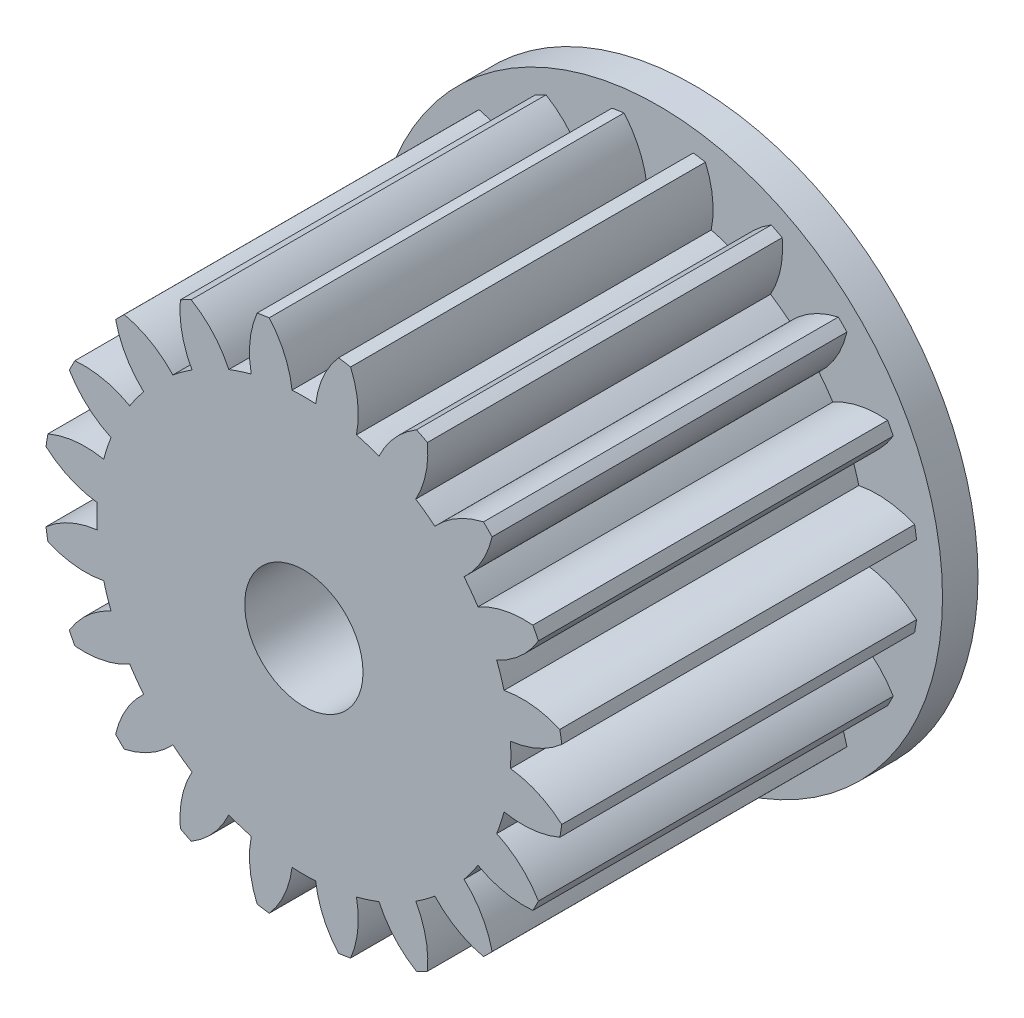
SolidWorks part; units mm, degrees
ref_plane "Front Plane" through (0, 0, 0) normal (0, 0, 1) x (1, 0, 0)
ref_plane "Top Plane" through (0, 0, 0) normal (0, 1, 0) x (1, 0, 0)
ref_plane "Right Plane" through (0, 0, 0) normal (1, 0, 0) x (0, 0, -1)
other "Configuration Table"
sketch "Sketch1" plane through (0, 0, 0) normal (0, 0, 1) x (1, 0, 0)
  circle A0 centre (0, 0) radius 12
  dimension "D1" = 24
extrude "Boss-Extrude1" add sketch "Sketch1" along normal blind 1.5
sketch "Sketch2" plane through (0, 0, 1.5) normal (0, 0, 1) x (1, 0, 0)
  arc A1 (-10.902, 1.5642) -> (-8.7347, 0.5992) centre (-8.2645, 4.5714) ccw
  arc A2 (-8.7347, 0.5992) -> (-8.7347, -0.4007) centre (0, 0.0992) ccw
  arc A3 (-8.7347, -0.4007) -> (-10.902, -1.3657) centre (-8.2645, -4.3729) ccw
  arc A4 (-10.902, -1.3657) -> (-10.8211, -1.8764) centre (0, 0.0992) ccw
  arc A5 (-10.8211, -1.8764) -> (-8.4617, -2.1245) centre (-9.242, 1.7987) ccw
  arc A6 (-8.4617, -2.1245) -> (-8.1527, -3.0754) centre (0, 0.0992) ccw
  arc A7 (-8.1527, -3.0754) -> (-9.9157, -4.6629) centre (-6.478, -6.7079) ccw
  arc A8 (-9.9157, -4.6629) -> (-9.681, -5.1236) centre (0, 0.0992) ccw
  arc A9 (-9.681, -5.1236) -> (-7.3604, -4.6304) centre (-9.3148, -1.1404) ccw
  arc A10 (-7.3604, -4.6304) -> (-6.7727, -5.4393) centre (0, 0.0992) ccw
  arc A11 (-6.7727, -5.4393) -> (-7.9588, -7.494) centre (-4.0574, -8.3766) ccw
  arc A12 (-7.9588, -7.494) -> (-7.5932, -7.8596) centre (0, 0.0992) ccw
  arc A13 (-7.5932, -7.8596) -> (-5.5386, -6.6734) centre (-8.4758, -3.9582) ccw
  arc A14 (-5.5386, -6.6734) -> (-4.7297, -7.2611) centre (0, 0.0992) ccw
  arc A15 (-4.7297, -7.2611) -> (-5.2229, -9.5817) centre (-1.2397, -9.2155) ccw
  arc A16 (-5.2229, -9.5817) -> (-4.7622, -9.8165) centre (0, 0.0992) ccw
  arc A17 (-4.7622, -9.8165) -> (-3.1746, -8.0535) centre (-6.8072, -6.3788) ccw
  arc A18 (-3.1746, -8.0535) -> (-2.2237, -8.3624) centre (0, 0.0992) ccw
  arc A19 (-2.2237, -8.3624) -> (-1.9757, -10.7219) centre (1.6994, -9.1427) ccw
  arc A20 (-1.9757, -10.7219) -> (-1.465, -10.8028) centre (0, 0.0992) ccw
  arc A21 (-1.465, -10.8028) -> (-0.4999, -8.6355) centre (-4.4722, -8.1652) ccw
  arc A22 (-0.4999, -8.6355) -> (0.4999, -8.6355) centre (0, 0.0992) ccw
  arc A23 (0.4999, -8.6355) -> (1.465, -10.8028) centre (4.4722, -8.1652) ccw
  arc A24 (1.465, -10.8028) -> (1.9757, -10.7219) centre (0, 0.0992) ccw
  arc A25 (1.9757, -10.7219) -> (2.2237, -8.3624) centre (-1.6994, -9.1427) ccw
  arc A26 (2.2237, -8.3624) -> (3.1746, -8.0535) centre (0, 0.0992) ccw
  arc A27 (3.1746, -8.0535) -> (4.7622, -9.8165) centre (6.8072, -6.3788) ccw
  arc A28 (4.7622, -9.8165) -> (5.2229, -9.5817) centre (0, 0.0992) ccw
  arc A29 (5.2229, -9.5817) -> (4.7297, -7.2611) centre (1.2397, -9.2155) ccw
  arc A30 (4.7297, -7.2611) -> (5.5386, -6.6734) centre (0, 0.0992) ccw
  arc A31 (5.5386, -6.6734) -> (7.5932, -7.8596) centre (8.4758, -3.9582) ccw
  arc A32 (7.5932, -7.8596) -> (7.9588, -7.494) centre (0, 0.0992) ccw
  arc A33 (7.9588, -7.494) -> (6.7727, -5.4393) centre (4.0574, -8.3766) ccw
  arc A34 (6.7727, -5.4393) -> (7.3604, -4.6304) centre (0, 0.0992) ccw
  arc A35 (7.3604, -4.6304) -> (9.681, -5.1236) centre (9.3148, -1.1404) ccw
  arc A36 (9.681, -5.1236) -> (9.9157, -4.6629) centre (0, 0.0992) ccw
  arc A37 (9.9157, -4.6629) -> (8.1527, -3.0754) centre (6.478, -6.7079) ccw
  arc A38 (8.1527, -3.0754) -> (8.4617, -2.1245) centre (0, 0.0992) ccw
  arc A39 (8.4617, -2.1245) -> (10.8211, -1.8764) centre (9.242, 1.7987) ccw
  arc A40 (10.8211, -1.8764) -> (10.902, -1.3657) centre (0, 0.0992) ccw
  arc A41 (10.902, -1.3657) -> (8.7347, -0.4007) centre (8.2645, -4.3729) ccw
  arc A42 (8.7347, -0.4007) -> (8.7347, 0.5992) centre (0, 0.0992) ccw
  arc A43 (8.7347, 0.5992) -> (10.902, 1.5642) centre (8.2645, 4.5714) ccw
  arc A44 (10.902, 1.5642) -> (10.8211, 2.0749) centre (0, 0.0992) ccw
  arc A45 (10.8211, 2.0749) -> (8.4617, 2.323) centre (9.242, -1.6002) ccw
  arc A46 (8.4617, 2.323) -> (8.1527, 3.2739) centre (0, 0.0992) ccw
  arc A47 (8.1527, 3.2739) -> (9.9157, 4.8614) centre (6.478, 6.9064) ccw
  arc A48 (9.9157, 4.8614) -> (9.681, 5.3221) centre (0, 0.0992) ccw
  arc A49 (9.681, 5.3221) -> (7.3604, 4.8289) centre (9.3148, 1.3389) ccw
  arc A50 (7.3604, 4.8289) -> (6.7727, 5.6378) centre (0, 0.0992) ccw
  arc A51 (6.7727, 5.6378) -> (7.9588, 7.6925) centre (4.0574, 8.5751) ccw
  arc A52 (7.9588, 7.6925) -> (7.5932, 8.0581) centre (0, 0.0992) ccw
  arc A53 (7.5932, 8.0581) -> (5.5386, 6.8719) centre (8.4758, 4.1567) ccw
  arc A54 (5.5386, 6.8719) -> (4.7297, 7.4596) centre (0, 0.0992) ccw
  arc A55 (4.7297, 7.4596) -> (5.2229, 9.7802) centre (1.2397, 9.414) ccw
  arc A56 (5.2229, 9.7802) -> (4.7622, 10.015) centre (0, 0.0992) ccw
  arc A57 (4.7622, 10.015) -> (3.1746, 8.252) centre (6.8072, 6.5773) ccw
  arc A58 (3.1746, 8.252) -> (2.2237, 8.5609) centre (0, 0.0992) ccw
  arc A59 (2.2237, 8.5609) -> (1.9757, 10.9204) centre (-1.6994, 9.3412) ccw
  arc A60 (1.9757, 10.9204) -> (1.465, 11.0013) centre (0, 0.0992) ccw
  arc A61 (1.465, 11.0013) -> (0.4999, 8.834) centre (4.4722, 8.3637) ccw
  arc A62 (0.4999, 8.834) -> (-0.4999, 8.834) centre (0, 0.0992) ccw
  arc A63 (-0.4999, 8.834) -> (-1.465, 11.0013) centre (-4.4722, 8.3637) ccw
  arc A64 (-1.465, 11.0013) -> (-1.9757, 10.9204) centre (0, 0.0992) ccw
  arc A65 (-1.9757, 10.9204) -> (-2.2237, 8.5609) centre (1.6994, 9.3412) ccw
  arc A66 (-2.2237, 8.5609) -> (-3.1746, 8.252) centre (0, 0.0992) ccw
  arc A67 (-3.1746, 8.252) -> (-4.7622, 10.015) centre (-6.8072, 6.5773) ccw
  arc A68 (-4.7622, 10.015) -> (-5.2229, 9.7802) centre (0, 0.0992) ccw
  arc A69 (-5.2229, 9.7802) -> (-4.7297, 7.4596) centre (-1.2397, 9.414) ccw
  arc A70 (-4.7297, 7.4596) -> (-5.5386, 6.8719) centre (0, 0.0992) ccw
  arc A71 (-5.5386, 6.8719) -> (-7.5932, 8.0581) centre (-8.4758, 4.1567) ccw
  arc A72 (-7.5932, 8.0581) -> (-7.9588, 7.6925) centre (0, 0.0992) ccw
  arc A73 (-7.9588, 7.6925) -> (-6.7727, 5.6378) centre (-4.0574, 8.5751) ccw
  arc A74 (-6.7727, 5.6378) -> (-7.3604, 4.8289) centre (0, 0.0992) ccw
  arc A75 (-7.3604, 4.8289) -> (-9.681, 5.3221) centre (-9.3148, 1.3389) ccw
  arc A76 (-9.681, 5.3221) -> (-9.9157, 4.8614) centre (0, 0.0992) ccw
  arc A77 (-9.9157, 4.8614) -> (-8.1527, 3.2739) centre (-6.478, 6.9064) ccw
  arc A78 (-8.1527, 3.2739) -> (-8.4617, 2.323) centre (0, 0.0992) ccw
  arc A79 (-8.4617, 2.323) -> (-10.8211, 2.0749) centre (-9.242, -1.6002) ccw
  arc A80 (-10.8211, 2.0749) -> (-10.902, 1.5642) centre (0, 0.0992) ccw
extrude "Boss-Extrude2" add sketch "Sketch2" along normal blind 15
sketch "Sketch3" plane through (0, 0, 16.5) normal (0, 0, 1) x (1, 0, 0)
  circle A0 centre (0, 0) radius 2.5
  dimension "D1" = 5
extrude "Cut-Extrude1" cut sketch "Sketch3" against normal blind 24
sketch "Sketch4" plane through (0, 0, 0) normal (0, 0, -1) x (-1, 0, 0)
  circle A0 centre (0, 0) radius 7
  dimension "D1" = 14
extrude "Cut-Extrude2" cut sketch "Sketch4" against normal blind 2
